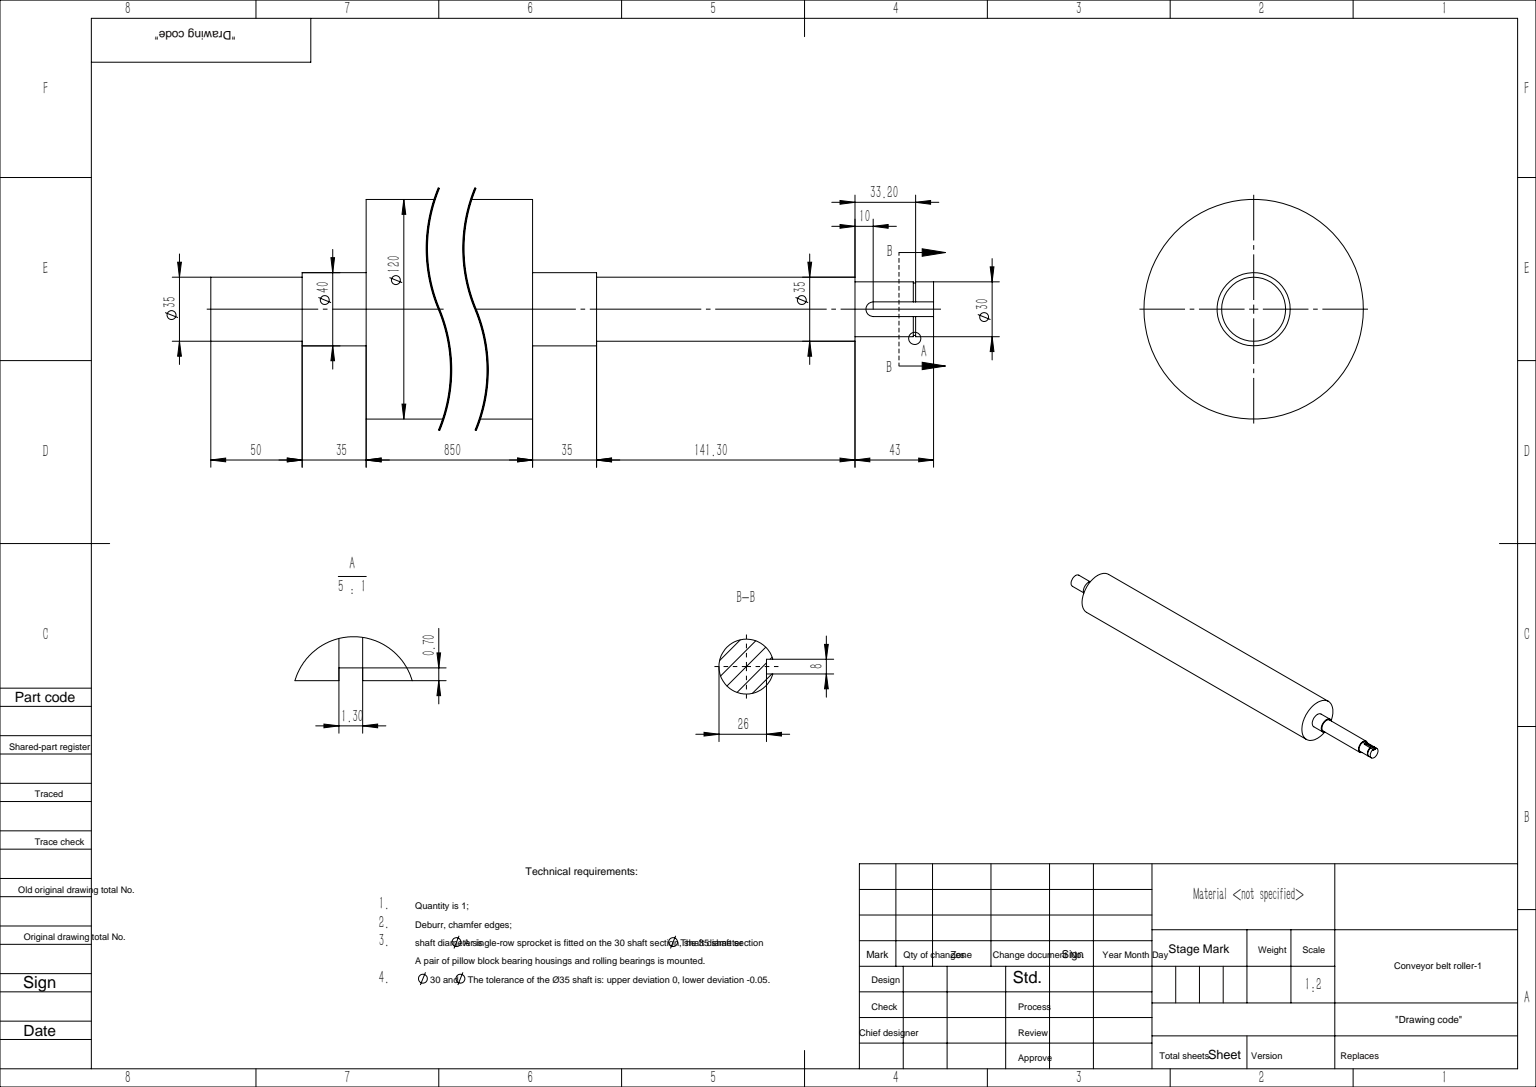
SolidWorks part; units mm, degrees
ref_plane "前视基准面" through (0, 0, 0) normal (0, 0, 1) x (1, 0, 0)
ref_plane "上视基准面" through (0, 0, 0) normal (0, 1, 0) x (1, 0, 0)
ref_plane "右视基准面" through (0, 0, 0) normal (1, 0, 0) x (0, 0, -1)
sketch "草图1" plane through (0, 0, 0) normal (0, 0, 1) x (1, 0, 0)
  line L0 (0, 0) -> (0, 17.5)
  line L1 (0, 17.5) -> (50, 17.5)
  line L2 (85, 20) -> (85, 60)
  line L3 (85, 60) -> (935, 60)
  line L4 (935, 60) -> (935, 20)
  line L5 (970, 17.5) -> (1111.3, 17.5)
  line L6 (1111.3, 17.5) -> (1111.3, 15)
  line L7 (1111.3, 15) -> (1154.3, 15)
  line L8 (1154.3, 15) -> (1154.3, 0)
  line L9 (1154.3, 0) -> (0, 0)
  line L10 (50, 17.5) -> (50, 20)
  line L11 (50, 20) -> (85, 20)
  line L12 (935, 20) -> (970, 20)
  line L13 (970, 20) -> (970, 17.5)
  dimension "D2" = 850
  dimension "D3" = 35
  dimension "D4" = 43
  dimension "D5" = 60
  dimension "D6" = 17.5
  dimension "D7" = 17.5
  dimension "D8" = 15
  dimension "D9" = 20
  dimension "D10" = 35
  dimension "D11" = 50
  dimension "D12" = 20
  dimension "D13" = 141.3
revolve "旋转1" add sketch "草图1" angle 360 about L9
ref_plane "基准面1" through (0, 15, 0) normal (0, 1, 0) x (1, 0, 0)
sketch "草图2" plane through (0, 15, 0) normal (0, 1, 0) x (1, 0, 0)
  line L0 (1111.3, 0) -> (1154.3, 0) construction
  line L1 (1111.3, -17.5) -> (1111.3, 17.5) construction
  line L2 (1154.3, -15) -> (1154.3, 15) construction
  line L3 (1111.3, -15) -> (1111.3, 15) construction
  line L4 (1121.3, 4) -> (1164.3, 4)
  line L5 (1121.3, -4) -> (1164.3, -4)
  line L6 (1164.3, 4) -> (1164.3, -4)
  arc A0 (1121.3, 4) -> (1121.3, -4) centre (1121.3, 0) ccw
  dimension "D1" = 10
  dimension "D3" = 4
  dimension "D2" = 10
extrude "切除-拉伸1" cut sketch "草图2" against normal blind 4
ref_plane "基准面2" through (1144.5, 0, 0) normal (1, 0, 0) x (0, 0, -1)
sketch "草图3" plane through (1144.5, 0, 0) normal (1, 0, 0) x (0, 0, -1)
  circle A0 centre (0, 0) radius 15
  circle A1 centre (0, 0) radius 14.3
  circle A2 centre (0, 0) radius 15 construction
  dimension "D1" = 28.6
extrude "切除-拉伸3" cut sketch "草图3" against normal blind 1.3
